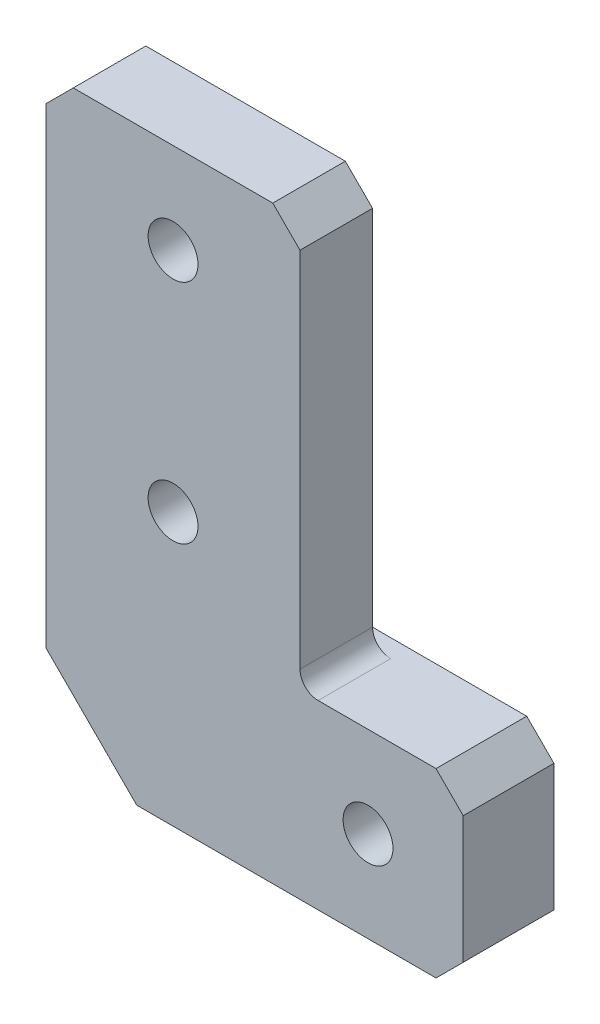
from build123d import *

# Parameters (mm, degrees)
SKETCH1_W           = 46
SKETCH1_H           = 65
BOSS_EXTRUDE1_DEPTH = 8
SKETCH2_R           = 2.75
CUT_EXTRUDE1_DEPTH  = 18
CHAMFER1_SIZE       = 10
SKETCH3_R           = 2.75
CUT_EXTRUDE2_DEPTH  = 10
SKETCH4_W           = 18
SKETCH4_H           = 45
CUT_EXTRUDE3_DEPTH  = 10
SKETCH5_R           = 2.75
BOSS_EXTRUDE2_DEPTH = 2
FILLET1_R           = 2
CHAMFER2_SIZE       = 3


with BuildPart() as part:
    # Sketch1 → Boss-Extrude1 (new body)
    with BuildSketch(Plane.XY):
        with Locations((-23, 32.5)):
            Rectangle(SKETCH1_W, SKETCH1_H)
    extrude(amount=BOSS_EXTRUDE1_DEPTH)

    # Sketch2 → Cut-Extrude1 (cut)
    with BuildSketch(Plane.XY.offset(8)):
        with Locations((-10.5, 10)):
            Circle(SKETCH2_R)
    extrude(amount=-CUT_EXTRUDE1_DEPTH, mode=Mode.SUBTRACT)

    # Chamfer1
    chamfer1_edges = [part.edges().sort_by_distance(p)[0] for p in [
        (-46, 0, 4),
    ]]
    chamfer(chamfer1_edges, length=CHAMFER1_SIZE)

    # Sketch3 → Cut-Extrude2 (cut)
    with BuildSketch(Plane.XY.offset(8)):
        with Locations((-32, 55)):
            Circle(SKETCH3_R)
        with Locations((-32, 30)):
            Circle(SKETCH3_R)
    extrude(amount=-CUT_EXTRUDE2_DEPTH, mode=Mode.SUBTRACT)

    # Sketch4 → Cut-Extrude3 (cut)
    with BuildSketch(Plane.XY.offset(8)):
        with Locations((-9, 42.5)):
            Rectangle(SKETCH4_W, SKETCH4_H)
    extrude(amount=-CUT_EXTRUDE3_DEPTH, mode=Mode.SUBTRACT)

    # Sketch5 → Boss-Extrude2 (add)
    with BuildSketch(Plane(origin=(0, 0, 0), x_dir=(-1, 0, 0), z_dir=(0, 0, -1))):
        Polygon((0, 20), (46, 20), (46, 10), (36, 0), (0, 0), align=None)
        with Locations(Location((10.5, 10, 0), (0, 0, 180))):
            Circle(SKETCH5_R, mode=Mode.SUBTRACT)
    extrude(amount=BOSS_EXTRUDE2_DEPTH)

    # Fillet1
    fillet1_edges = [part.edges().sort_by_distance(p)[0] for p in [
        (-18, 20, 4),
    ]]
    fillet(fillet1_edges, radius=FILLET1_R)

    # Chamfer2
    chamfer2_edges = [part.edges().sort_by_distance(p)[0] for p in [
        (0, 0, 3),
        (0, 20, 3),
        (-18, 65, 4),
        (-46, 65, 4),
    ]]
    chamfer(chamfer2_edges, length=CHAMFER2_SIZE)


solid = part.part
